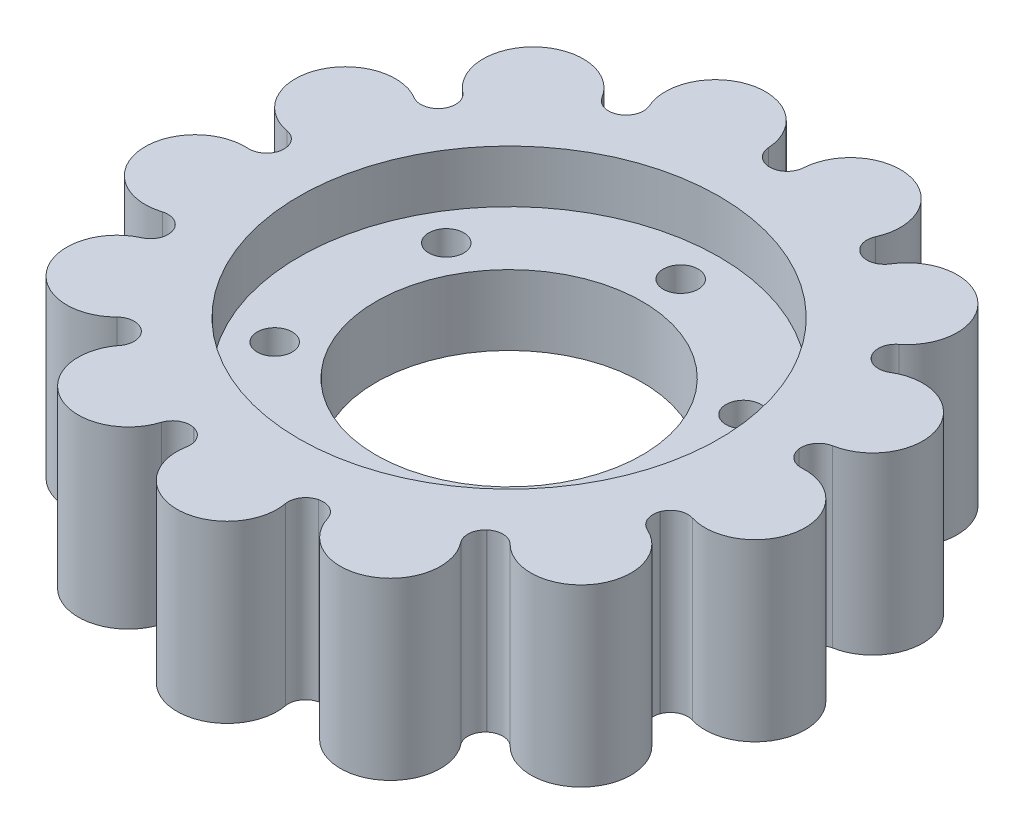
SolidWorks part; units mm, degrees
material "EPDM 60 硬度计"
ref_plane "前视基准面" through (0, 0, 0) normal (0, 0, 1) x (1, 0, 0)
ref_plane "上视基准面" through (0, 0, 0) normal (0, 1, 0) x (1, 0, 0)
ref_plane "右视基准面" through (0, 0, 0) normal (1, 0, 0) x (0, 0, -1)
sketch "草图2" plane through (0, 0, 0) normal (0, 1, 0) x (1, 0, 0)
  arc A0 (0, 74.39) -> (-34.6049, 65.8511) centre (0, 0) ccw
  arc A2 (-4.9901, 79.0751) -> (0, 74.39) centre (0, 79.39) ccw
  arc A14 (-34.6049, 65.8511) -> (-32.3096, 72.2922) centre (-36.894, 70.2963) ccw
  arc A26 (-4.9904, 79.0751) -> (-32.3096, 72.2922) centre (-19.2683, 78.174) ccw
  arc A27 (-4.9901, 79.0751) -> (-4.9904, 79.0751) centre (0, 0) ccw
  arc A51 (23.782, -75.6232) -> (23.7695, -75.5829) centre (18.9994, -77.0816) ccw [skipped]
  arc A52 (62.2806, 49.0568) -> (67.9119, 40.8136) centre (65.3362, 45.0991) ccw [skipped]
  arc A53 (77.8348, 14.4741) -> (79.1, 4.5786) centre (78.8106, 9.5702) ccw [skipped]
  arc A54 (75.642, -23.3543) -> (72.1673, -32.7054) centre (74.2305, -28.151) ccw [skipped]
  arc A58 (56.1284, -55.8359) -> (48.7019, -62.4971) centre (52.6451, -59.4229) ccw [skipped]
  arc A59 (-14.0786, -77.9715) -> (-23.7689, -75.5831) centre (-18.9988, -77.0817) ccw [skipped]
  arc A60 (-48.7014, -62.4975) -> (-56.1407, -55.8487) centre (-52.6445, -59.4231) ccw [skipped]
  arc A61 (-72.1671, -32.7059) -> (-75.6476, -23.3564) centre (-74.23, -28.1513) ccw [skipped]
  arc A62 (-79.1, 4.5783) -> (-77.8312, 14.473) centre (-78.8103, 9.5699) ccw [skipped]
  arc A63 (-67.9119, 40.8134) -> (-62.1932, 48.9876) centre (-65.336, 45.0988) ccw [skipped]
  arc A71 (32.3292, 72.3366) -> (41.1662, 67.6987) centre (36.8941, 70.2965) ccw [skipped]
extrude "凸台-拉伸1" add sketch "草图2" along normal mid plane 50 contours A2 A27 A26 A14 A0
sketch "草图3" plane through (0, 0, 0) normal (0, 1, 0) x (1, 0, 0)
  circle A0 centre (0, 0) radius 74.39
  circle A1 centre (0, 0) radius 60
extrude "凸台-拉伸2" add sketch "草图3" along normal mid plane 50
pattern_circular "阵列(圆周)1" count 13 over 360 about axis through (0, 0, 0) along (0, 1, 0) of "凸台-拉伸1"
sketch "草图4" plane through (0, 0, 0) normal (0, 1, 0) x (1, 0, 0)
  line L0 (3.981, 0) -> (50003.981, 0) construction
  line L1 (0, 3.5138) -> (0, 50003.5138) construction
  line L2 (0, 0) -> (43301.2702, 25000) construction
  line L3 (0, 0) -> (43301.2702, -25000) construction
  circle A0 centre (0, 0) radius 60
  circle A1 centre (0, 0) radius 38
  circle A2 centre (0, 0) radius 49 construction
  circle A3 centre (0, 49) radius 5
  circle A4 centre (42.4352, 24.5) radius 5
  circle A5 centre (42.4352, -24.5) radius 5
  circle A6 centre (0, -49) radius 5
  circle A7 centre (-42.4352, -24.5) radius 5
  circle A8 centre (-42.4352, 24.5) radius 5
  point P27 (0, 0)
  dimension "D1" = 30
  dimension "D2" = 30
extrude "凸台-拉伸3" add sketch "草图4" along normal mid plane 20
